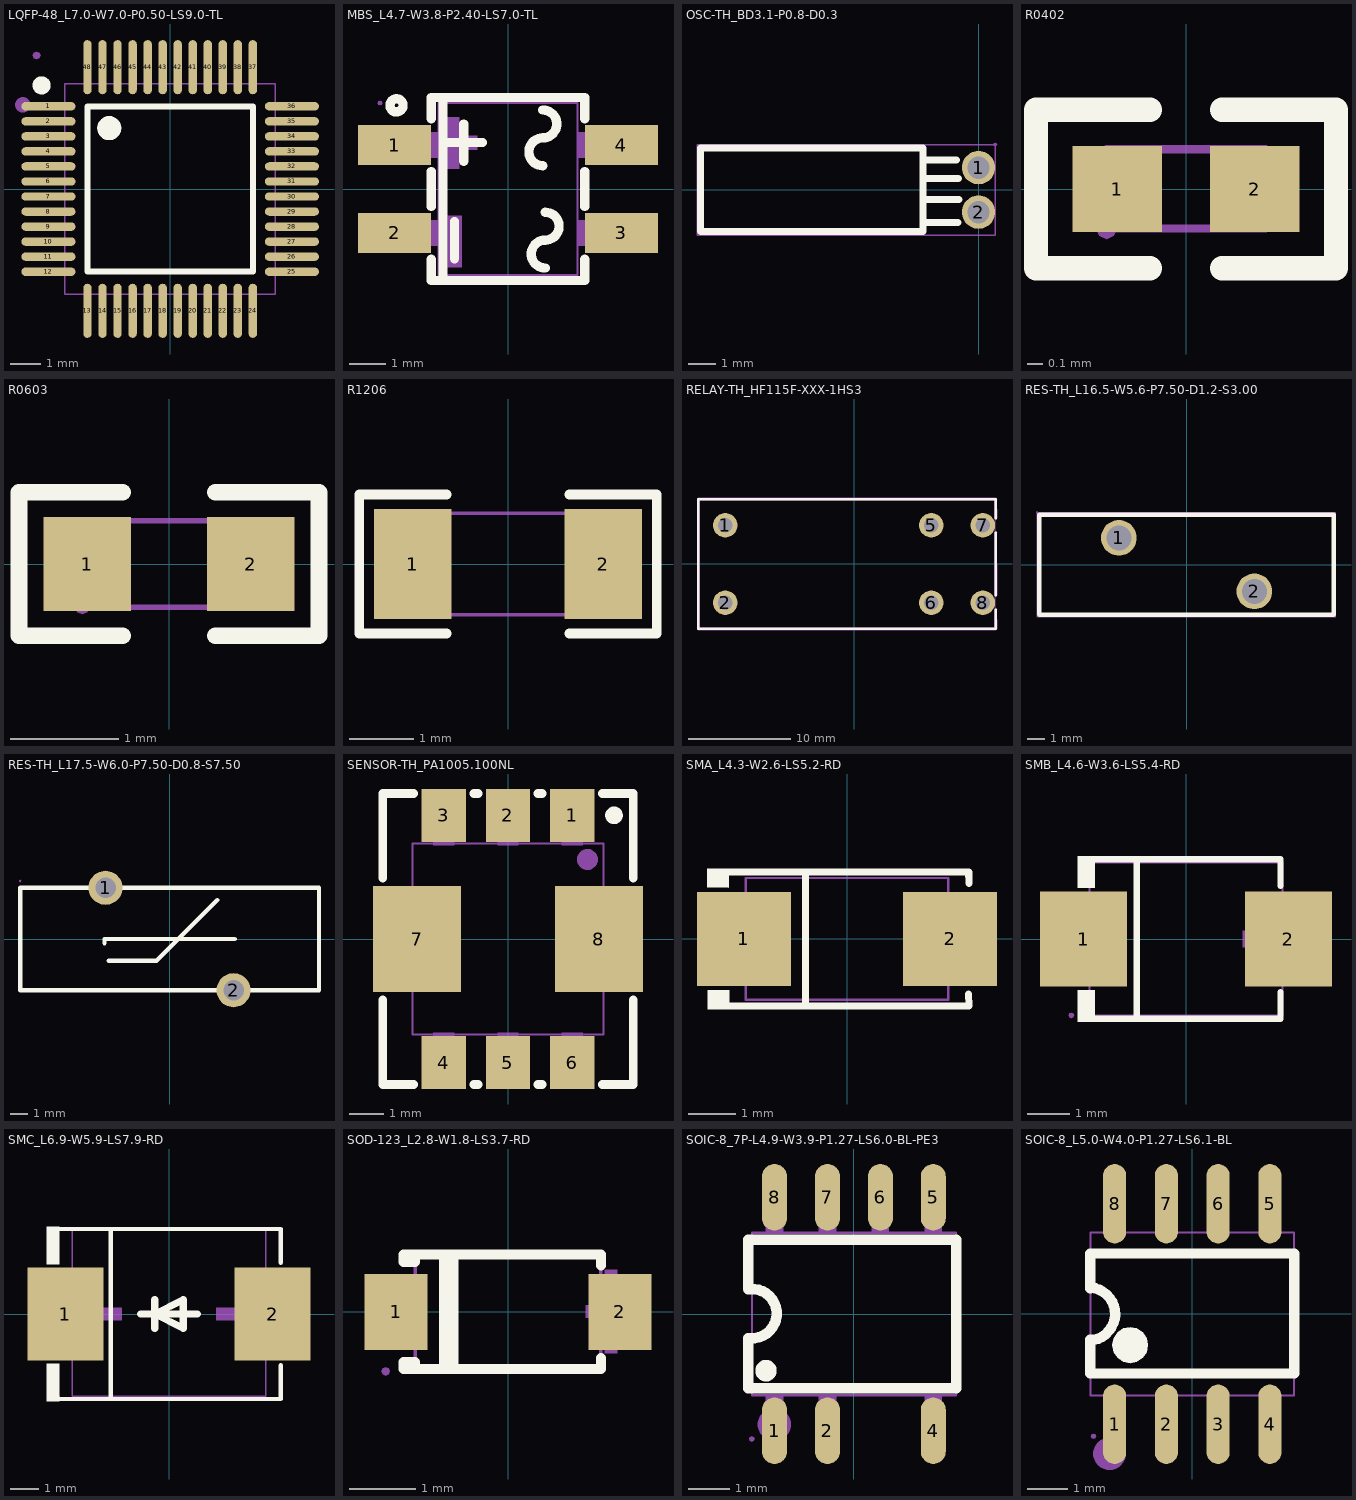
[diagram p0: the footprints below, top view; thin cyan lines are the x and y axes]
# Altium footprint library MISC84429-11.PcbLib: 64 footprints (part 3 of 4)
Each footprint in its own frame and in the unit in brackets; x right, y up, seen from the top. Pads: shape width x height; smd on the part's side, far side on the other; paste and mask are expansions set on the pad; w line width, h text height; cw(c..) or ccw(c..) is an arc to the next point about the centre after c.

## LQFP-48_L7.0-W7.0-P0.50-LS9.0-TL [mm]
pads (48):
  oval 1.8x0.28 smd: 1(-4.05,2.75) 2(-4.05,2.25) 3(-4.05,1.75) 4(-4.05,1.25) 5(-4.05,0.75) 6(-4.05,0.25) 7(-4.05,-0.25) 8(-4.05,-0.75) 9(-4.05,-1.25) 10(-4.05,-1.75) 11(-4.05,-2.25) 12(-4.05,-2.75) 25(4.05,-2.75) 26(4.05,-2.25) 27(4.05,-1.75) 28(4.05,-1.25) 29(4.05,-0.75) 30(4.05,-0.25) 31(4.05,0.25) 32(4.05,0.75) 33(4.05,1.25) 34(4.05,1.75) 35(4.05,2.25) 36(4.05,2.75)
  oval 0.28x1.8 smd: 13(-2.75,-4.05) 14(-2.25,-4.05) 15(-1.75,-4.05) 16(-1.25,-4.05) 17(-0.75,-4.05) 18(-0.25,-4.05) 19(0.25,-4.05) 20(0.75,-4.05) 21(1.25,-4.05) 22(1.75,-4.05) 23(2.25,-4.05) 24(2.75,-4.05) 37(2.75,4.05) 38(2.25,4.05) 39(1.75,4.05) 40(1.25,4.05) 41(0.75,4.05) 42(0.25,4.05) 43(-0.25,4.05) 44(-0.75,4.05) 45(-1.25,4.05) 46(-1.75,4.05) 47(-2.25,4.05) 48(-2.75,4.05)
Top Overlay:
  lines w0.2: -2.75,-2.75 2.75,-2.75 2.75,2.75 -2.75,2.75 -2.75,-2.75
  lines w0.3: -4.125,3.447 cw(c-4.275,3.448) -4.125,3.449
  lines w0.4: -1.826,2.022 cw(c-2.026,2.023) -1.826,2.024
Mechanical 1:
  circle w0.254: c-4.9,2.8 r0.127
Mechanical 2:
  drawing of 101 lines, arcs and shapes, not listed

## MBS_L4.7-W3.8-P2.40-LS7.0-TL [mm]
pads (4):
  rect 2x1.1 smd: 1(-3.1,1.2) 2(-3.1,-1.2) 3(3.1,-1.2) 4(3.1,1.2)
Top Overlay:
  circle w0.254: c-3.048,2.286 r0.18
  lines w0.254: -2.1,-1.921 -2.1,-2.5 2.1,-2.5 2.1,-1.921 ; -2.1,-0.479 -2.1,0.479 ; -2.1,1.921 -2.1,2.5 2.1,2.5 2.1,1.921 ; -1.777,-2.5 -1.777,2.5 ; -1.715,1.27 -0.699,1.27 ; -1.461,-1.905 -1.461,-0.889 ; -1.207,0.762 -1.207,1.778 ; 0.952,0.635 cw(c0.952,1.016) 0.952,1.397 ccw(c0.952,1.778) 0.952,2.159 ; 1.016,-2.159 cw(c1.016,-1.778) 1.016,-1.397 ccw(c1.016,-1.016) 1.016,-0.635 ; 2.1,-0.479 2.1,0.479
Mechanical 1:
  region: -2.232,1.078 -2.232,1.459 -0.835,1.459 -0.835,1.078
  region: -1.331,0.559 -1.712,0.559 -1.712,1.956 -1.331,1.956
  region: -1.269,-2.133 -1.65,-2.133 -1.65,-0.736 -1.269,-0.736
Mechanical 2:
  region: -3.435,2.35 -3.454,2.304 -3.5,2.285 -3.546,2.304 -3.565,2.35 -3.546,2.396 -3.5,2.415 -3.454,2.396
  region: -2.61,-1.55 -2.61,-0.85 -1.89,-0.85 -1.89,-1.55
  region: -3.5,-1.55 -3.5,-0.85 -2.6,-0.85 -2.6,-1.55
  region: -2.61,0.85 -2.61,1.55 -1.89,1.55 -1.89,0.85
  region: -3.5,0.85 -3.5,1.55 -2.6,1.55 -2.6,0.85
  region: 1.89,0.85 1.89,1.55 2.61,1.55 2.61,0.85
  region: 2.6,0.85 2.6,1.55 3.5,1.55 3.5,0.85
  region: 1.89,-1.55 1.89,-0.85 2.61,-0.85 2.61,-1.55
  region: 2.6,-1.55 2.6,-0.85 3.5,-0.85 3.5,-1.55
  lines w0.051: -1.9,-2.35 -1.9,2.35 1.9,2.35 1.9,-2.35 -1.9,-2.35

## OSC-TH_BD3.1-P0.8-D0.3 [mm]
pads (2):
  round 1.2 hole 0.8: 1(0,0.8) 2(0,-0.8)
Top Overlay:
  lines w0.254: -2,-1.177 -0.74,-1.177 ; -2,-0.35 -0.698,-0.35 ; -2,0.403 -0.73,0.403 ; -2,1.071 -0.786,1.071 ; -10,-1.5 -2,-1.5 -2,1.5 -10,1.5 -10,-1.5
Mechanical 2:
  region: 0.665,1.627 0.646,1.581 0.6,1.562 0.554,1.581 0.535,1.627 0.554,1.673 0.6,1.692 0.646,1.673
  region: 0.306,-0.8 0.283,-0.917 0.216,-1.016 0.117,-1.083 0,-1.106 -0.117,-1.083 -0.216,-1.016 -0.283,-0.917 -0.306,-0.8 -0.283,-0.683 -0.216,-0.584 -0.117,-0.518 0,-0.494 0.117,-0.518 0.216,-0.584 0.283,-0.683
  region: 0.306,0.8 0.283,0.683 0.216,0.584 0.117,0.517 0,0.494 -0.117,0.517 -0.216,0.584 -0.283,0.683 -0.306,0.8 -0.283,0.917 -0.216,1.016 -0.117,1.083 0,1.106 0.117,1.083 0.216,1.016 0.283,0.917
  lines w0.051: -10.127,-1.627 -10.127,1.627 0.6,1.627 0.6,-1.627 -10.127,-1.627

## R0402 [mm]
pads (2):
  rect 0.566x0.54 smd paste-100 mask+0.051: 1(-0.433,0) 2(0.433,0)
Top Overlay:
  lines w0.152: -0.226,-0.499 -0.944,-0.499 -0.944,0.499 -0.226,0.499 ; 0.226,-0.499 0.944,-0.499 0.944,0.499 0.226,0.499
Top Paste:
  region: 0.135,-0.23 0.135,0.23 0.175,0.27 0.676,0.27 0.716,0.23 0.716,-0.23 0.676,-0.27 0.175,-0.27
  region: -0.135,-0.23 -0.135,0.23 -0.175,0.27 -0.676,0.27 -0.716,0.23 -0.716,-0.23 -0.676,-0.27 -0.175,-0.27
Mechanical 2:
  region: -0.435,-0.25 -0.454,-0.296 -0.5,-0.315 -0.546,-0.296 -0.565,-0.25 -0.546,-0.204 -0.5,-0.185 -0.454,-0.204
  region: 0.251,-0.25 0.251,0.25 0.501,0.25 0.501,-0.25
  region: -0.249,0.25 -0.249,-0.25 -0.499,-0.25 -0.499,0.25
  lines w0.051: -0.5,-0.25 -0.5,0.25 0.5,0.25 0.5,-0.25 -0.5,-0.25

## R0603 [mm]
pads (2):
  rect 0.806x0.864 smd paste-100 mask+0.051: 1(-0.753,0) 2(0.753,0)
Top Overlay:
  lines w0.152: -0.426,-0.661 -1.385,-0.661 -1.385,0.661 -0.426,0.661 ; 0.426,-0.661 1.385,-0.661 1.385,0.661 0.426,0.661
Top Paste:
  region: -1.195,-0.45 -0.395,-0.45 -0.345,-0.4 -0.345,-0.172 -0.715,-0.172 -0.715,0.158 -0.345,0.158 -0.345,0.4 -0.395,0.45 -1.195,0.45 -1.245,0.4 -1.245,-0.4
  region: 1.195,0.45 0.395,0.45 0.345,0.4 0.345,0.172 0.715,0.172 0.715,-0.158 0.345,-0.158 0.345,-0.4 0.395,-0.45 1.195,-0.45 1.245,-0.4 1.245,0.4
Mechanical 15:
  region: 0.8,-0.4 0.8,0.4 0.5,0.4 0.5,-0.4
  region: -0.8,-0.4 -0.8,0.4 -0.5,0.4 -0.5,-0.4
  region: -0.735,-0.4 -0.754,-0.446 -0.8,-0.465 -0.846,-0.446 -0.865,-0.4 -0.846,-0.354 -0.8,-0.335 -0.754,-0.354
  lines w0.051: -0.8,-0.4 0.8,-0.4 0.8,0.4 -0.8,0.4 -0.8,-0.4

## R1206 [mm]
pads (2):
  rect 1.208x1.701 smd paste-100 mask+0.051: 1(-1.479,0) 2(1.479,0)
Top Overlay:
  lines w0.152: -0.951,-1.079 -2.311,-1.079 -2.311,1.079 -0.951,1.079 ; 0.951,-1.079 2.311,-1.079 2.311,1.079 0.951,1.079
Top Paste:
  region: 0.875,-0.75 0.875,-0.389 0.975,-0.289 1.186,-0.289 1.286,-0.189 1.286,0.189 1.186,0.289 0.975,0.289 0.875,0.389 0.875,0.75 0.975,0.85 1.983,0.85 2.083,0.75 2.083,-0.75 1.983,-0.85 0.975,-0.85
  region: -0.875,-0.75 -0.875,-0.389 -0.975,-0.289 -1.186,-0.289 -1.286,-0.189 -1.286,0.189 -1.186,0.289 -0.975,0.289 -0.875,0.389 -0.875,0.75 -0.975,0.85 -1.983,0.85 -2.083,0.75 -2.083,-0.75 -1.983,-0.85 -0.975,-0.85
Mechanical 2:
  region: -1.485,-0.787 -1.504,-0.833 -1.55,-0.852 -1.596,-0.833 -1.615,-0.787 -1.596,-0.742 -1.55,-0.722 -1.504,-0.742
  region: -1.55,-0.788 -1.55,0.788 -1.1,0.788 -1.1,-0.788
  region: 1.55,-0.788 1.55,0.788 1.1,0.788 1.1,-0.788
  lines w0.051: -1.55,-0.788 -1.55,0.788 1.55,0.788 1.55,-0.788 -1.55,-0.788

## RELAY-TH_HF115F-XXX-1HS3 [mm]
pads (6):
  round 2.4 hole 1.4 paste+0 mask-0.45: 1(-12.6,3.78) 2(-12.6,-3.78) 5(7.56,3.78) 6(7.56,-3.78) 7(12.6,3.78) 8(12.6,-3.78)
Top Overlay:
  lines w0.254: 13.843,-4.486 13.843,-6.35 -15.24,-6.35 -15.24,6.35 13.843,6.35 13.843,4.486 ; 13.843,-3.073 13.843,3.073
Mechanical 1:
  region: 13.716,4.486 13.716,6.223 -15.24,6.212 -15.338,6.253 -15.378,6.35 -15.338,6.447 -15.24,6.487 -15.24,6.477 13.843,6.487 13.94,6.447 13.98,6.35 13.97,6.35 13.98,4.486 13.94,4.388 13.843,4.348 13.745,4.388 13.705,4.486
  region: -15.113,6.35 -15.113,-6.223 13.716,-6.223 13.705,-4.486 13.745,-4.389 13.843,-4.349 13.94,-4.389 13.98,-4.486 13.97,-4.486 13.98,-6.35 13.94,-6.447 13.843,-6.488 13.843,-6.477 -15.24,-6.488 -15.338,-6.447 -15.378,-6.35 -15.367,-6.35 -15.378,6.35 -15.338,6.447 -15.24,6.487 -15.143,6.447 -15.103,6.35
  region: 13.716,-3.073 13.705,3.073 13.745,3.17 13.843,3.21 13.94,3.17 13.98,3.073 13.97,3.073 13.98,-3.073 13.94,-3.171 13.843,-3.211 13.745,-3.171 13.705,-3.073
Mechanical 2:
  region: -15.135,6.35 -15.154,6.304 -15.2,6.285 -15.246,6.304 -15.265,6.35 -15.246,6.396 -15.2,6.415 -15.154,6.396
  region: -12.85,-3.53 -12.35,-3.53 -12.35,-4.03 -12.85,-4.03
  region: -12.85,4.029 -12.35,4.029 -12.35,3.529 -12.85,3.529
  region: 7.31,-3.38 7.81,-3.38 7.81,-4.18 7.31,-4.18
  region: 12.35,-3.38 12.85,-3.38 12.85,-4.18 12.35,-4.18
  region: 7.31,4.18 7.81,4.18 7.81,3.38 7.31,3.38
  region: 12.35,4.18 12.85,4.18 12.85,3.38 12.35,3.38
  lines w0.051: -15.2,-6.35 -15.2,6.35 13.8,6.35 13.8,-6.35 -15.2,-6.35

## RES-TH_L16.5-W5.6-P7.50-D1.2-S3.00 [mm]
pads (2):
  round 2 hole 1.4: 1(-3.8,1.5) 2(3.8,-1.5)
Top Overlay:
  lines w0.254: -8.25,-2.8 8.25,-2.8 8.25,2.8 -8.25,2.8 -8.25,-2.8
Mechanical 2:
  region: -3.188,1.5 -3.235,1.266 -3.368,1.067 -3.566,0.935 -3.8,0.888 -4.034,0.935 -4.233,1.067 -4.365,1.266 -4.412,1.5 -4.365,1.734 -4.233,1.933 -4.034,2.065 -3.8,2.112 -3.566,2.065 -3.368,1.933 -3.235,1.734
  region: 4.412,-1.5 4.365,-1.734 4.233,-1.933 4.034,-2.065 3.8,-2.112 3.566,-2.065 3.368,-1.933 3.235,-1.734 3.188,-1.5 3.235,-1.266 3.368,-1.067 3.566,-0.935 3.8,-0.888 4.034,-0.935 4.233,-1.067 4.365,-1.266
  region: -8.312,2.927 -8.331,2.881 -8.377,2.862 -8.423,2.881 -8.442,2.927 -8.423,2.973 -8.377,2.992 -8.331,2.973
  lines w0.051: -8.377,-2.927 8.377,-2.927 8.377,2.927 -8.377,2.927 -8.377,-2.927

## RES-TH_L17.5-W6.0-P7.50-D0.8-S7.50 [mm]
pads (2):
  round 2 hole 1.2 paste+0 mask-0.35: 1(-3.749,3) 2(3.749,-3)
Top Overlay:
  lines w0.254: -3.81,-0.254 -3.81,0 3.81,0 ; -3.556,-1.27 -0.762,-1.27 2.794,2.286 ; -8.75,-3 -8.75,3 8.75,3 8.75,-3 -8.75,-3
Mechanical 2:
  region: -8.685,3.4 -8.704,3.354 -8.75,3.335 -8.796,3.354 -8.815,3.4 -8.796,3.446 -8.75,3.465 -8.704,3.446
  region: -3.341,3 -3.372,2.844 -3.461,2.712 -3.593,2.623 -3.749,2.592 -3.905,2.623 -4.037,2.712 -4.126,2.844 -4.157,3 -4.126,3.156 -4.037,3.288 -3.905,3.377 -3.749,3.408 -3.593,3.377 -3.461,3.288 -3.372,3.156
  region: 4.157,-3 4.126,-3.156 4.037,-3.288 3.905,-3.377 3.749,-3.408 3.593,-3.377 3.461,-3.288 3.372,-3.156 3.341,-3 3.372,-2.844 3.461,-2.712 3.593,-2.623 3.749,-2.592 3.905,-2.623 4.037,-2.712 4.126,-2.844
  lines w0.051: -8.75,-3 -8.75,3 8.75,3 8.75,-3 -8.75,-3

## SENSOR-TH_PA1005.100NL [mm]
pads (8):
  rect 1.27x1.52 smd: 1(1.85,3.555) 2(0,3.555) 3(-1.85,3.555) 4(-1.85,-3.555) 5(0,-3.555) 6(1.85,-3.555)
  rect 2.54x3.05 smd: 7(-2.615,0) 8(2.615,0)
Top Overlay:
  circle w0.254: c3.048,3.556 r0.127
  lines w0.254: -3.605,-1.756 -3.605,-4.19 -2.716,-4.19 ; -3.605,1.756 -3.605,4.19 -2.716,4.19 ; -0.984,-4.19 -0.866,-4.19 ; -0.984,4.19 -0.866,4.19 ; 0.866,-4.19 0.984,-4.19 ; 0.866,4.19 0.984,4.19 ; 2.716,-4.19 3.605,-4.19 3.605,-1.756 ; 2.716,4.19 3.605,4.19 ; 3.605,1.756 3.605,4.19 ; 3.605,4.19 3.605,4.19
Mechanical 1:
  circle w0.3: c2.286,2.286 r0.15
Mechanical 2:
  region: 3.669,4.2 3.65,4.154 3.604,4.135 3.558,4.154 3.539,4.2 3.558,4.246 3.604,4.265 3.65,4.246
  region: 1.55,2.7 1.55,3.71 2.15,3.71 2.15,2.7
  region: 1.55,3.7 1.55,4.2 2.15,4.2 2.15,3.7
  region: -0.3,3.7 -0.3,4.2 0.3,4.2 0.3,3.7
  region: -2.15,3.7 -2.15,4.2 -1.55,4.2 -1.55,3.7
  region: -2.15,-4.2 -2.15,-3.7 -1.55,-3.7 -1.55,-4.2
  region: -0.3,-4.2 -0.3,-3.7 0.3,-3.7 0.3,-4.2
  region: 1.55,-4.2 1.55,-3.7 2.15,-3.7 2.15,-4.2
  region: 2.604,1.2 3.604,1.2 3.604,-1.2 2.604,-1.2
  region: -2.604,-1.201 -3.604,-1.201 -3.604,1.199 -2.604,1.199
  region: -0.3,2.7 -0.3,3.71 0.3,3.71 0.3,2.7
  region: -2.15,2.7 -2.15,3.71 -1.55,3.71 -1.55,2.7
  region: 2.15,-2.7 2.15,-3.71 1.55,-3.71 1.55,-2.7
  region: 0.3,-2.7 0.3,-3.71 -0.3,-3.71 -0.3,-2.7
  region: -1.55,-2.7 -1.55,-3.71 -2.15,-3.71 -2.15,-2.7
  lines w0.051: -2.75,-2.75 -2.75,2.75 2.75,2.75 2.75,-2.75 -2.75,-2.75

## SMA_L4.3-W2.6-LS5.2-RD [mm]
pads (2):
  rect 2x2 smd: 1(-2.2,0) 2(2.2,0)
Top Overlay:
  region: -2.52,1.502 -2.521,1.096 -2.981,1.1 -2.977,1.502
  region: -2.512,-1.096 -2.513,-1.503 -2.973,-1.498 -2.969,-1.096
  lines w0.152: -2.596,-1.426 2.596,-1.426 ; -2.596,1.426 2.596,1.426 2.603,1.187 ; -0.884,-1.426 -0.884,1.426 ; 2.593,-1.176 2.6,-1.415
Mechanical 1:
  region: -2.317,-0.101 -2.317,0.101 -1.507,0.101 -1.507,-0.101
  region: 2.29,-0.09 2.29,0.112 1.48,0.112 1.48,-0.09
  region: 2.014,-0.675 2.014,0.675 1.811,0.675 1.811,-0.675
Mechanical 2:
  region: -2.54,-1.3 -2.559,-1.346 -2.605,-1.365 -2.651,-1.346 -2.67,-1.3 -2.651,-1.254 -2.605,-1.235 -2.559,-1.254
  region: 2.605,0.725 2.605,-0.725 1.48,-0.725 1.48,0.725
  region: -1.48,0.725 -1.48,-0.725 -2.605,-0.725 -2.605,0.725
  lines w0.051: -2.16,-1.3 -2.16,1.3 2.16,1.3 2.16,-1.3 -2.16,-1.3

## SMB_L4.6-W3.6-LS5.4-RD [mil]
pads (2):
  rect 80.61x88.23 smd: 1(-95,0) 2(95,0)
Top Overlay:
  region: -84.65,76.87 -84.65,47.53 -100.39,47.53 -100.39,76.87
  region: -84.65,-76.87 -84.65,-47.53 -100.39,-47.53 -100.39,-76.87
  lines w6: -87.65,-73.87 87.65,-73.87 87.65,-49.54 ; -87.65,73.87 87.65,73.87 87.65,49.54 ; -45.78,-73.87 -45.78,73.87
Mechanical 1:
  region: -125,7.5 -55,7.5 -55,-7.5 -125,-7.5
  region: 52.5,7.5 122.5,7.5 122.5,-7.5 52.5,-7.5
  region: 80,-35 80,35 95,35 95,-35
Mechanical 2:
  region: -103.74,-70.87 -104.49,-72.68 -106.3,-73.43 -108.11,-72.68 -108.86,-70.87 -108.11,-69.06 -106.3,-68.31 -104.49,-69.06
  region: 106.3,40.35 106.3,-40.35 61.71,-40.35 61.71,40.35
  region: -106.3,40.35 -106.3,-40.35 -61.71,-40.35 -61.71,40.35
  lines w2: -89.57,-70.87 89.57,-70.87 89.57,70.87 -89.57,70.87 -89.57,-70.87

## SMC_L6.9-W5.9-LS7.9-RD [mm]
pads (2):
  rect 2.7x3.3 smd: 1(-3.686,0) 2(3.686,0)
Top Overlay:
  region: -3.9,3.102 -3.9,1.772 -4.357,1.772 -4.357,3.102
  region: -3.9,-3.102 -3.9,-1.772 -4.357,-1.772 -4.357,-3.102
  lines w0.152: -3.976,-3.026 3.976,-3.026 3.976,-1.823 ; -3.976,3.026 3.976,3.026 3.976,1.823 ; -2.069,-3.026 -2.069,3.026
  lines w0.254: -1.016,0 1.016,0 ; -0.508,0.508 -0.508,-0.508 -0.508,0 ; -0.508,0 0.508,-0.508 0.508,0.508 -0.508,0
Mechanical 1:
  region: -3.457,-0.221 -3.457,0.221 -1.687,0.221 -1.687,-0.221
  region: 3.457,-0.221 3.457,0.221 1.687,0.221 1.687,-0.221
  region: 2.794,-1.475 2.794,1.475 2.351,1.475 2.351,-1.475
Mechanical 2:
  region: -3.885,-2.95 -3.904,-2.996 -3.95,-3.015 -3.996,-2.996 -4.015,-2.95 -3.996,-2.904 -3.95,-2.885 -3.904,-2.904
  region: -3.95,-1.5 -3.95,1.5 -2.7,1.5 -2.7,-1.5
  region: 3.95,-1.5 3.95,1.5 2.7,1.5 2.7,-1.5
  lines w0.051: -3.45,-2.921 -3.45,2.979 3.45,2.979 3.45,-2.921 -3.45,-2.921

## SOD-123_L2.8-W1.8-LS3.7-RD [mm]
pads (2):
  rect 0.95x1.15 smd: 1(-1.692,0) 2(1.692,0)
Top Overlay:
  lines w0.152: -0.97,-0.866 -0.97,0.866 ; -0.827,-0.866 -0.827,0.866 ; 1.406,-0.698 1.406,-0.866 -1.406,-0.866 ; 1.406,0.698 1.406,0.866 -1.406,0.866 ; -1.406,-0.866 -1.58,-0.866 -1.58,-0.755 -1.406,-0.755 -1.406,-0.866 ; -1.406,0.866 -1.58,0.866 -1.58,0.755 -1.406,0.755 -1.406,0.866
Mechanical 1:
  region: -2.03,0.095 -2.03,-0.095 -1.272,-0.095 -1.272,0.095
  region: 1.935,0.098 1.935,-0.092 1.177,-0.092 1.177,0.098
  region: 1.651,0.635 1.651,-0.629 1.461,-0.629 1.461,0.635
Mechanical 2:
  region: -1.785,-0.9 -1.804,-0.946 -1.85,-0.965 -1.896,-0.946 -1.915,-0.9 -1.896,-0.854 -1.85,-0.835 -1.804,-0.854
  region: -1.851,-0.465 -1.851,0.465 -1.301,0.465 -1.301,-0.465
  region: 1.851,-0.465 1.851,0.465 1.301,0.465 1.301,-0.465
  lines w0.051: -1.4,-0.9 -1.4,0.9 1.4,0.9 1.4,-0.9 -1.4,-0.9

## SOIC-8_7P-L4.9-W3.9-P1.27-LS6.0-BL-PE3 [mm]
pads (7):
  oval 0.6x1.6 smd: 1(-1.905,-2.8) 2(-0.635,-2.8) 4(1.905,-2.8) 5(1.905,2.8) 6(0.635,2.8) 7(-0.635,2.8) 8(-1.905,2.8)
Top Overlay:
  circle w0.254: c-2.11,-1.36 r0.13
  lines w0.254: -2.54,-0.58 -2.54,-1.778 2.46,-1.778 2.46,1.778 -2.54,1.778 -2.54,0.6 ; -2.49,-0.58 ccw(c-2.445,0.01) -2.49,0.6
Mechanical 1:
  circle w0.4: c-1.91,-2.65 r0.2
Mechanical 2:
  region: -2.385,-3 -2.404,-3.046 -2.45,-3.065 -2.496,-3.046 -2.515,-3 -2.496,-2.954 -2.45,-2.935 -2.404,-2.954
  region: -2.11,-2.26 -2.11,-1.94 -1.7,-1.94 -1.7,-2.26
  region: -2.11,-3 -2.11,-2.25 -1.7,-2.25 -1.7,-3
  region: -0.84,-2.26 -0.84,-1.94 -0.43,-1.94 -0.43,-2.26
  region: -0.84,-3 -0.84,-2.25 -0.43,-2.25 -0.43,-3
  region: 1.7,-2.26 1.7,-1.94 2.11,-1.94 2.11,-2.26
  region: 1.7,-3 1.7,-2.25 2.11,-2.25 2.11,-3
  region: -2.11,1.94 -2.11,2.26 -1.7,2.26 -1.7,1.94
  region: -2.11,2.25 -2.11,3 -1.7,3 -1.7,2.25
  region: -0.84,1.94 -0.84,2.26 -0.43,2.26 -0.43,1.94
  region: -0.84,2.25 -0.84,3 -0.43,3 -0.43,2.25
  region: 0.43,1.94 0.43,2.26 0.84,2.26 0.84,1.94
  region: 0.43,2.25 0.43,3 0.84,3 0.84,2.25
  region: 1.7,1.94 1.7,2.26 2.11,2.26 2.11,1.94
  region: 1.7,2.25 1.7,3 2.11,3 2.11,2.25
  lines w0.051: -2.45,-1.95 2.45,-1.95 2.45,1.95 -2.45,1.95 -2.45,-1.95

## SOIC-8_L5.0-W4.0-P1.27-LS6.1-BL [mil]
pads (8):
  oval 22.38x76.78 smd: 1(-75,-106.5) 2(-25,-106.5) 3(25,-106.5) 4(75,-106.5) 5(75,106.5) 6(25,106.5) 7(-25,106.5) 8(-75,106.5)
Top Overlay:
  region: -77.21,-30
  region: -77.21,-30 -77.24,-29.87 -75.92,-23.27 -72.19,-17.68 -66.6,-13.95 -60,-12.63 -53.4,-13.95 -47.81,-17.68 -44.08,-23.27 -42.76,-29.87 -42.79,-30 -42.76,-30.13 -44.08,-36.73 -47.81,-42.32 -53.4,-46.05 -60,-47.37 -66.6,-46.05 -72.19,-42.32 -75.92,-36.73 -77.24,-30.13
  region: -42.79,-30
  lines w10: -98.42,-25 -98.42,-57.51 98.42,-57.51 98.42,58.41 -98.42,58.41 -98.42,25 ; -95,-25 ccw(c-100,0) -93.82,24.73
Mechanical 1:
  circle w15.75: c-80,-135 r7.87
Mechanical 2:
  region: -92.73,-118.11 -93.47,-119.92 -95.28,-120.67 -97.09,-119.92 -97.84,-118.11 -97.09,-116.31 -95.28,-115.56 -93.47,-116.31
  region: -83.07,-118.11 -83.07,-85.24 -66.93,-85.24 -66.93,-118.11
  region: -83.07,-85.63 -83.07,-76.38 -66.93,-76.38 -66.93,-85.63
  region: -33.07,-118.11 -33.07,-85.24 -16.93,-85.24 -16.93,-118.11
  region: -33.07,-85.63 -33.07,-76.38 -16.93,-76.38 -16.93,-85.63
  region: 16.93,-118.11 16.93,-85.24 33.07,-85.24 33.07,-118.11
  region: 16.93,-85.63 16.93,-76.38 33.07,-76.38 33.07,-85.63
  region: 66.93,-118.11 66.93,-85.24 83.07,-85.24 83.07,-118.11
  region: 66.93,-85.63 66.93,-76.38 83.07,-76.38 83.07,-85.63
  region: -83.07,85.24 -83.07,118.11 -66.93,118.11 -66.93,85.24
  region: -83.07,76.38 -83.07,85.63 -66.93,85.63 -66.93,76.38
  region: -33.07,85.24 -33.07,118.11 -16.93,118.11 -16.93,85.24
  region: -33.07,76.38 -33.07,85.63 -16.93,85.63 -16.93,76.38
  region: 16.93,85.24 16.93,118.11 33.07,118.11 33.07,85.24
  region: 16.93,76.38 16.93,85.63 33.07,85.63 33.07,76.38
  region: 66.93,85.24 66.93,118.11 83.07,118.11 83.07,85.24
  region: 66.93,76.38 66.93,85.63 83.07,85.63 83.07,76.38
  lines w2: -98.43,-78.74 -98.43,78.74 98.42,78.74 98.42,-78.74 -98.43,-78.74